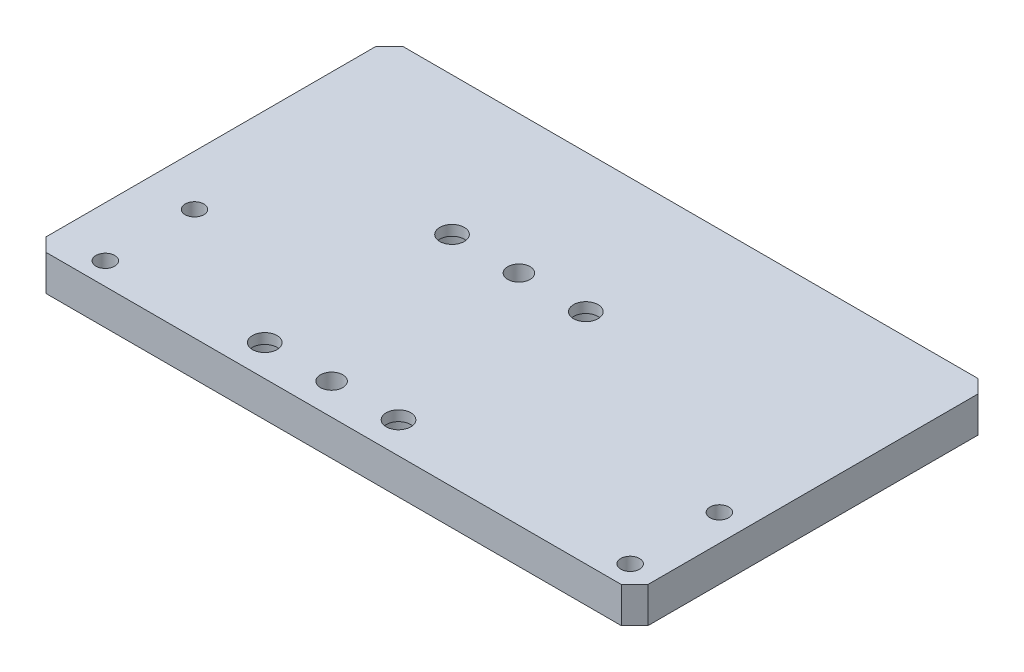
from build123d import *

# Parameters (mm, degrees)
SKETCH1_W                                            = 135
SKETCH1_H                                            = 80
BOSS_EXTRUDE1_DEPTH                                  = 8
CBORE_FOR_M5_HEXAGON_SOCKET_HEAD_CAP_SCR_D           = 5.5
CBORE_FOR_M5_HEXAGON_SOCKET_HEAD_CAP_SCR_CBORE_D     = 10
CBORE_FOR_M5_HEXAGON_SOCKET_HEAD_CAP_SCR_CBORE_DEPTH = 5.7
M5_TAPPED_HOLE1_D                                    = 4.2
CHAMFER1_SIZE                                        = 3
F_5_0MM_DOWEL_HOLE1_D                                = 5


with BuildPart() as part:
    # Sketch1 → Boss-Extrude1 (new body)
    with BuildSketch(Plane(origin=(0, 0, 0), x_dir=(1, 0, 0), z_dir=(0, 1, 0))):
        with Locations((67.5, 40)):
            Rectangle(SKETCH1_W, SKETCH1_H)
    extrude(amount=BOSS_EXTRUDE1_DEPTH)

    # CBORE for M5 Hexagon socket head cap screws1 (through all)
    with Locations(Plane(origin=(0, 0, 0), x_dir=(-1, 0, 0), z_dir=(0, -1, 0))):
        with Locations((-75.05, 49), (-45.05, 49), (-45.05, 7), (-75.05, 7)):
            CounterBoreHole(CBORE_FOR_M5_HEXAGON_SOCKET_HEAD_CAP_SCR_D / 2, CBORE_FOR_M5_HEXAGON_SOCKET_HEAD_CAP_SCR_CBORE_D / 2, CBORE_FOR_M5_HEXAGON_SOCKET_HEAD_CAP_SCR_CBORE_DEPTH)

    # M5 Tapped Hole1 (through all)
    with Locations(Plane(origin=(0, 8, 0), x_dir=(1, 0, 0), z_dir=(0, 1, 0))):
        with Locations((129, 25), (129, 5), (11.3, 25), (11.3, 5)):
            Hole(M5_TAPPED_HOLE1_D / 2)

    # Chamfer1
    chamfer1_edges = [part.edges().sort_by_distance(p)[0] for p in [
        (0, 4, -80),
        (135, 4, -80),
        (135, 4, 0),
        (0, 4, 0),
    ]]
    chamfer(chamfer1_edges, length=CHAMFER1_SIZE)

    # Ø5.0mm Dowel Hole1 (through all)
    with Locations(Plane(origin=(0, 0, 0), x_dir=(-1, 0, 0), z_dir=(0, -1, 0))):
        with Locations((-60.05, 7), (-60.05, 49)):
            Hole(F_5_0MM_DOWEL_HOLE1_D / 2)


solid = part.part
